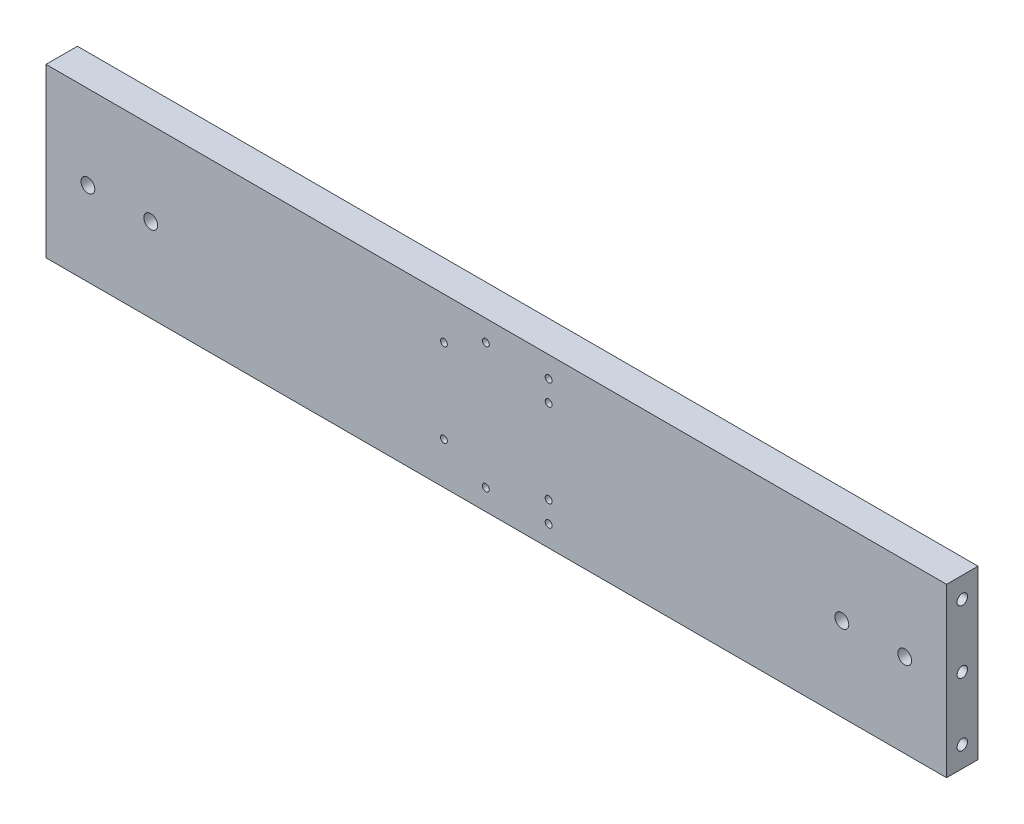
from build123d import *

# Parameters (mm, degrees)
SKETCH_1_W                   = 430
SKETCH_1_H                   = 80
EXTRUDE_1_DEPTH              = 15
HOLE_WIZARD_M4_6_D           = 3.3
HOLE_WIZARD_M4_7_D           = 3.3
HOLE_WIZARD_M4_5_D           = 6.6
HOLE_WIZARD_M4_5_CBORE_D     = 11
HOLE_WIZARD_M4_5_CBORE_DEPTH = 6.4
HOLE_WIZARD_M6_1_AT_2_COUNT  = 2
HOLE_WIZARD_M6_1_AT_2_PITCH  = 30
HOLE_WIZARD_M6_1_AT_3_COUNT  = 2
HOLE_WIZARD_M6_1_AT_3_PITCH  = 60


with BuildPart() as part:
    # 草图1 → 凸台-拉伸1 (new body)
    with BuildSketch(Plane.XY):
        Rectangle(SKETCH_1_W, SKETCH_1_H)
    extrude(amount=EXTRUDE_1_DEPTH)

    # M4 螺纹孔6 (through all)
    with Locations(Plane(origin=(0, 0, 0), x_dir=(1, 0, 0), z_dir=(0, 0, -1))):
        with Locations((25, 20), (-25, 20), (-25, -20), (25, -20)):
            Hole(HOLE_WIZARD_M4_6_D / 2)

    # M4 螺纹孔7 (through all)
    with Locations(Plane(origin=(0, 0, 0), x_dir=(-1, 0, 0), z_dir=(0, 0, -1))):
        with Locations((5, 30), (5, -30), (-25, 30), (-25, -30)):
            Hole(HOLE_WIZARD_M4_7_D / 2)

    # M4 六角凹头螺钉的柱形沉头孔5 (through all)
    with Locations(Plane(origin=(0, 0, 0), x_dir=(-1, 0, 0), z_dir=(0, 0, -1))):
        with Locations((-195, 0), (-165, 0), (165, 0), (195, 0)):
            CounterBoreHole(HOLE_WIZARD_M4_5_D / 2, HOLE_WIZARD_M4_5_CBORE_D / 2, HOLE_WIZARD_M4_5_CBORE_DEPTH)

    # 草图35 → M6 螺纹孔1 (revolve, cut)
    with BuildSketch(Plane(origin=(215, 30, 7.5), x_dir=(0, 0, -1), z_dir=(0, 1, 0))):
        Polygon((0, 0), (0, 21.502151548), (2.5, 20), (2.5, 0), align=None)
    hole_wizard_m6_1 = revolve(axis=Axis((221.35, 30, 7.5), (-1, 0, 0)), mode=Mode.SUBTRACT)

    # M6 螺纹孔1 at 2: M6 螺纹孔1 ×2
    with Locations(*[(0, -i * HOLE_WIZARD_M6_1_AT_2_PITCH, 0) for i in range(1, HOLE_WIZARD_M6_1_AT_2_COUNT)]):
        add(hole_wizard_m6_1, mode=Mode.SUBTRACT)

    # M6 螺纹孔1 at 3: M6 螺纹孔1 ×2
    with Locations(*[(0, -i * HOLE_WIZARD_M6_1_AT_3_PITCH, 0) for i in range(1, HOLE_WIZARD_M6_1_AT_3_COUNT)]):
        add(hole_wizard_m6_1, mode=Mode.SUBTRACT)

    # 镜向1: M6 螺纹孔1 across plane
    add(hole_wizard_m6_1.mirror(Plane(origin=(0, 0, 0), x_dir=(0, 0, 1), z_dir=(1, 0, 0))), mode=Mode.SUBTRACT)

    # 镜向1 copy 1 sketch → 镜向1 copy 1 (revolve, cut)
    with BuildSketch(Plane(origin=(-215, 0, 7.5), x_dir=(0, 0, -1), z_dir=(0, 1, 0))):
        Polygon((0, 0), (0, -21.502151548), (2.5, -20), (2.5, 0), align=None)
    revolve(axis=Axis((-221.35, 0, 7.5), (-1, 0, 0)), mode=Mode.SUBTRACT)

    # 镜向1 copy 2 sketch → 镜向1 copy 2 (revolve, cut)
    with BuildSketch(Plane(origin=(-215, -30, 7.5), x_dir=(0, 0, -1), z_dir=(0, 1, 0))):
        Polygon((0, 0), (0, -21.502151548), (2.5, -20), (2.5, 0), align=None)
    revolve(axis=Axis((-221.35, -30, 7.5), (-1, 0, 0)), mode=Mode.SUBTRACT)


solid = part.part
